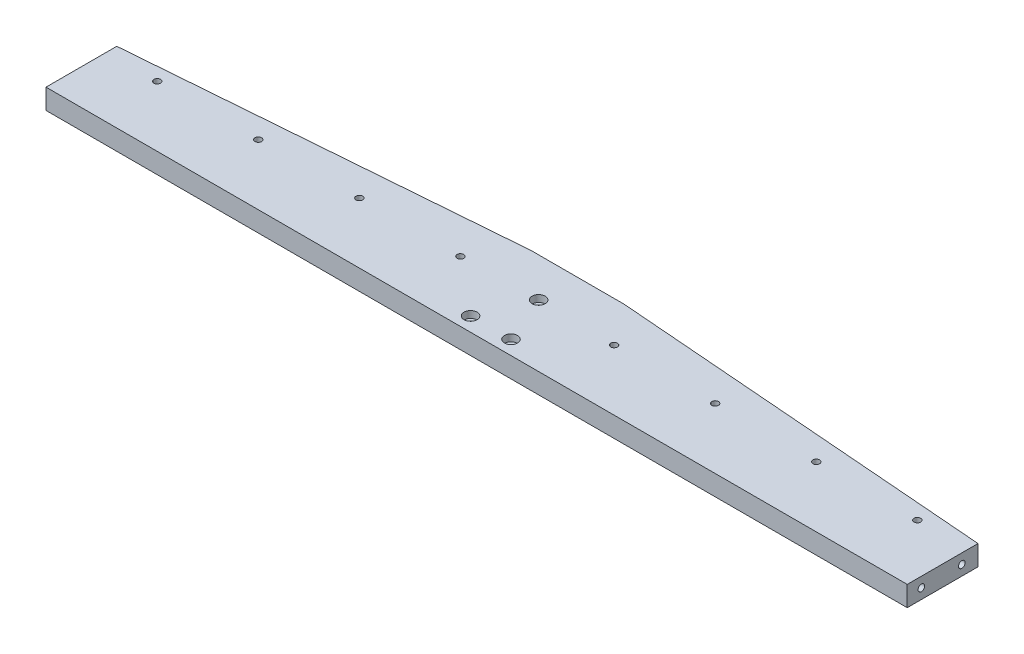
SolidWorks part; units mm, degrees
material "A6061"
ref_plane "前视" through (0, 0, 0) normal (0, 0, 1) x (1, 0, 0)
ref_plane "上视" through (0, 0, 0) normal (0, 1, 0) x (1, 0, 0)
ref_plane "右视" through (0, 0, 0) normal (1, 0, 0) x (0, 0, -1)
sketch "草图1" plane through (0, 0, 0) normal (0, 1, 0) x (1, 0, 0)
  line L1 (-213, -25) -> (213, -25)
  line L2 (-213, -25) -> (-213, 25)
  line L3 (-213, 25) -> (213, 25)
  line L4 (213, -25) -> (213, 25)
  line L5 (-213, -25) -> (213, 25) construction
  line L6 (-213, 25) -> (213, -25) construction
  point P0 (0, 0)
  dimension "D1" = 426
  dimension "D2" = 50
extrude "凸台-拉伸1" add sketch "草图1" along normal blind 10
hole_wizard "M4 螺纹孔1" positions "草图2" profile "草图3" tap size "M4" standard "GB"
sketch "草图2" plane through (-213, 0, 0) normal (-1, 0, 0) x (0, 0, 1)
  line L0 (25, 10) -> (25, 0) construction
  point P0 (-2, 5)
  point P2 (18, 5)
  point P10 (25, 5)
  dimension "D1" = 20
  dimension "D2" = 7
sketch "草图3" plane through (-213, 5, -2) normal (0, 1, 0) x (0, 0, 1)
  line L0 (0, 0) -> (0, 12.4914)
  line L1 (0, 12.4914) -> (1.65, 11.5)
  line L2 (1.65, 11.5) -> (1.65, 0)
  line L5 (1.65, 0) -> (0, 0)
  line L10 (0, 12.4914) -> (-1.65, 11.5) construction
  line L11 (0, -6.35) -> (0, 107.95) construction
  dimension "螺纹孔钻头直径" = 3.3
  dimension "螺纹孔钻头深度" = 11.5
  dimension "导头角度" = 118
cosmetic thread "孔螺蚊线1" parameters "D1"=8, "D2"=4
cosmetic thread "孔螺蚊线2" parameters "D1"=8, "D2"=4
mirror "镜向1" about plane through (0, 0, 0) normal (1, 0, 0) of "M4 螺纹孔1"
hole_wizard "M3 六角凹头螺钉的柱形沉头孔1" positions "草图7" profile "草图8" counterbore size "M3" standard "ISO" end condition through all
sketch "草图7" plane through (0, 10, 0) normal (0, 1, 0) x (1, 0, 0)
  line L0 (10, -18) -> (-10, -18) construction
  line L3 (0, -18) -> (0, -25)
  line L4 (-213, -25) -> (213, -25) construction
  line L7 (0, -18) -> (0, 5.7) construction
  point P0 (10, -18)
  point P3 (-10, -18)
  point P12 (0, 5.7)
  dimension "D1" = 20
  dimension "D2" = 23.7
  dimension "D3" = 7
sketch "草图8" plane through (10, 10, 18) normal (1, 0, 0) x (0, 0, 1)
  line L0 (0, 0) -> (0, 10)
  line L1 (0, 10) -> (1.7, 10)
  line L3 (1.7, 10) -> (1.7, 3.4)
  line L4 (1.7, 3.4) -> (3.25, 3.4)
  line L5 (3.25, 3.4) -> (3.25, 0)
  line L7 (3.25, 0) -> (0, 0)
  line L11 (0, -6.35) -> (0, 107.95) construction
  dimension "通孔孔直径" = 3.4
  dimension "通孔孔深度" = 10
  dimension "柱形沉头孔直径" = 6.5
  dimension "柱形沉头孔深度" = 3.4
hole_wizard "M4 螺纹孔2" positions "草图9" profile "草图10" tap size "M4" standard "ISO" end condition through all
sketch "草图9" plane through (0, 10, 0) normal (0, 1, 0) x (1, 0, 0)
  line L0 (-213, 25) -> (-213, -25) construction
  line L1 (-213, -25) -> (213, -25) construction
  point P0 (-38, 5)
  point P2 (-88, 5)
  point P4 (-138, 5)
  point P8 (-188, 5)
  dimension "D1" = 25
  dimension "D2" = 50
  dimension "D3" = 50
  dimension "D4" = 50
  dimension "D5" = 30
sketch "草图10" plane through (-38, 10, -5) normal (1, 0, 0) x (0, 0, 1)
  line L0 (0, 0) -> (0, 10)
  line L1 (0, 10) -> (1.65, 10)
  line L2 (1.65, 10) -> (1.65, 0)
  line L5 (1.65, 0) -> (0, 0)
  line L11 (0, -6.35) -> (0, 107.95) construction
  dimension "通孔螺纹孔钻头直径" = 3.3
  dimension "通孔螺纹孔钻头深度" = 10
cosmetic thread "孔螺蚊线3" parameters "D2"=4
cosmetic thread "孔螺蚊线4" parameters "D2"=4
cosmetic thread "孔螺蚊线5" parameters "D2"=4
cosmetic thread "孔螺蚊线6" parameters "D2"=4
mirror "镜向2" about plane through (0, 0, 0) normal (1, 0, 0) of "M4 螺纹孔2"
chamfer "倒角1" distance 15 distance2 190 1 edges at (213, 5, -25)
chamfer "倒角2" distance 190 distance2 15 1 edges at (-213, 5, -25)
